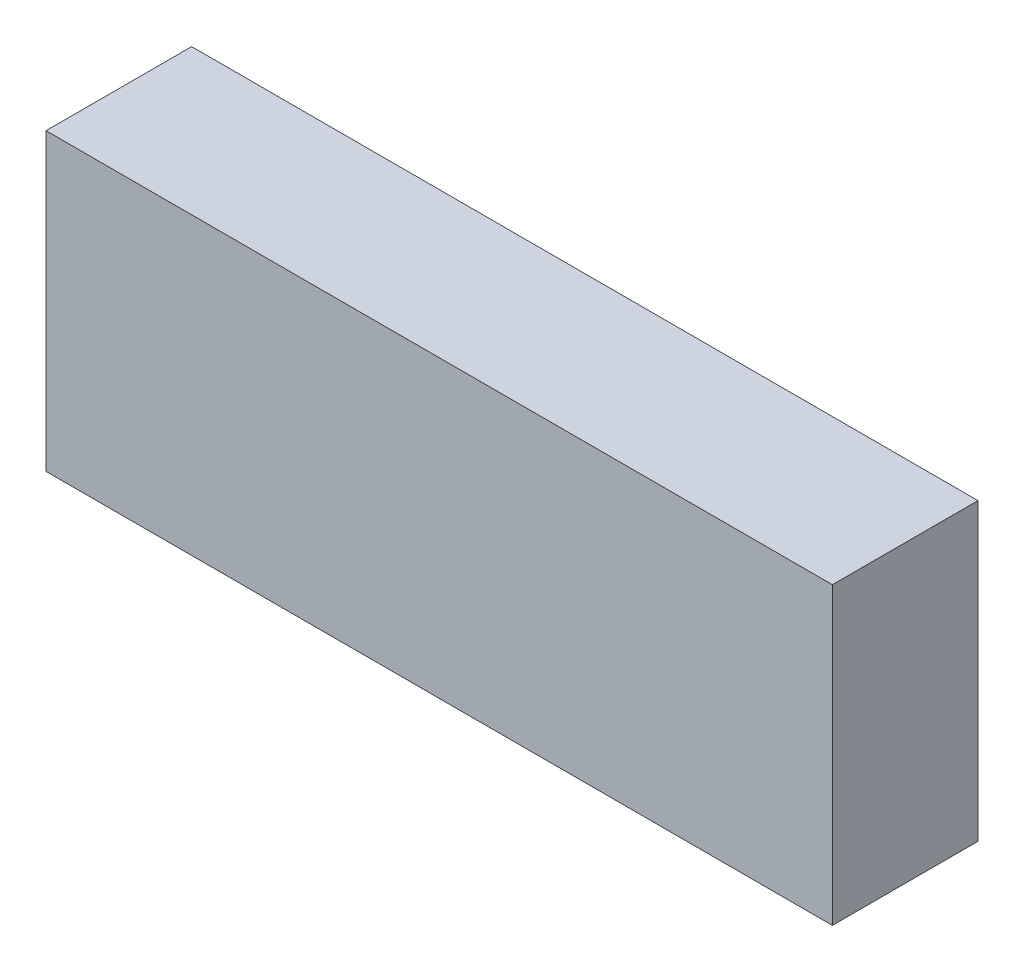
SolidWorks part; units mm, degrees
ref_plane "Front Plane" through (0, 0, 0) normal (0, 0, 1) x (1, 0, 0)
ref_plane "Top Plane" through (0, 0, 0) normal (0, 1, 0) x (1, 0, 0)
ref_plane "Right Plane" through (0, 0, 0) normal (1, 0, 0) x (0, 0, -1)
other "Configuration Table"
sketch "Sketch2" plane through (0, 0, 0) normal (0, 0, 1) x (1, 0, 0)
  line L0 (165, 827.602) -> (-165, 827.602) construction
  line L1 (125, 733.801) -> (-125, 733.801)
  line L2 (125, 733.801) -> (125, 827.602)
  line L3 (125, 827.602) -> (-125, 827.602)
  line L4 (-125, 733.801) -> (-125, 827.602)
  line L5 (-125, 797.602) -> (-125, 577.4627) construction
extrude "Boss-Extrude1" add sketch "Sketch2" along normal blind 44
other "Move Face1" face at (0, 780.7015, 44) parameters "D1"=2.3
